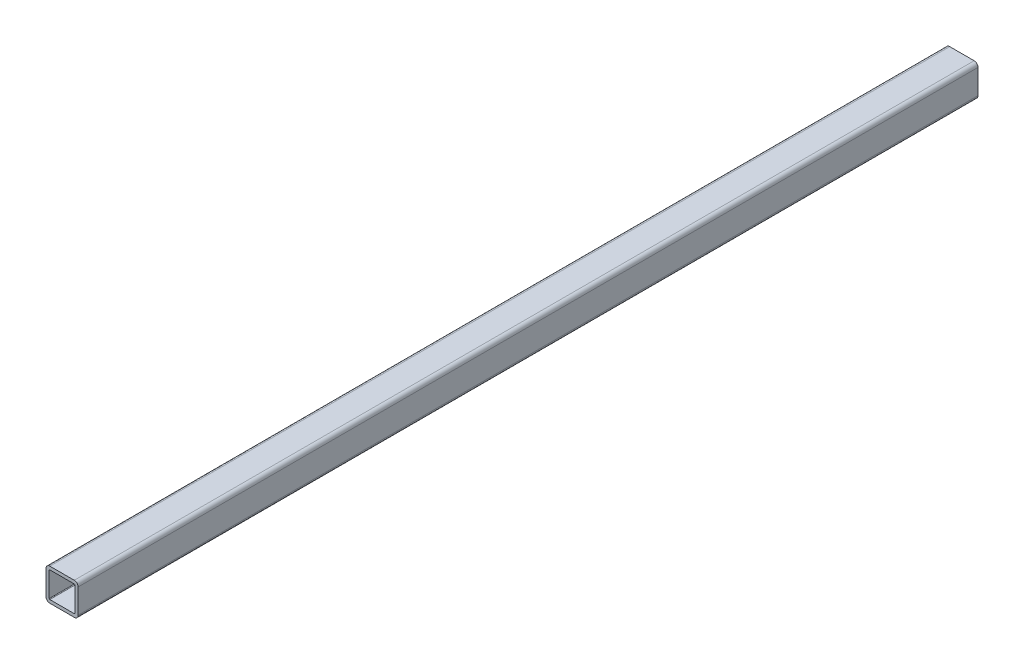
from build123d import *

# Parameters (mm, degrees)
BOSS_EXTRUDE1_DEPTH = 1400


with BuildPart() as part:
    # Sketch1 → Boss-Extrude1 (new body)
    with BuildSketch(Plane.XY):
        with BuildLine():
            Line((6, 0), (44, 0))
            ThreePointArc((44, 0), (48.242640687, 1.757359313), (50, 6))
            Line((50, 6), (50, 44))
            ThreePointArc((50, 44), (48.242640687, 48.242640687), (44, 50))
            Line((44, 50), (6, 50))
            ThreePointArc((6, 50), (1.757359313, 48.242640687), (0, 44))
            Line((0, 44), (0, 6))
            ThreePointArc((0, 6), (1.757359313, 1.757359313), (6, 0))
        make_face()
        with BuildLine():
            Line((6, 45), (44, 45))
            ThreePointArc((44, 45), (44.707106781, 44.707106781), (45, 44))
            Line((45, 44), (45, 6))
            ThreePointArc((45, 6), (44.707106781, 5.292893219), (44, 5))
            Line((44, 5), (6, 5))
            ThreePointArc((6, 5), (5.292893219, 5.292893219), (5, 6))
            Line((5, 6), (5, 44))
            ThreePointArc((5, 44), (5.292893219, 44.707106781), (6, 45))
        make_face(mode=Mode.SUBTRACT)
    extrude(amount=BOSS_EXTRUDE1_DEPTH)


solid = part.part
